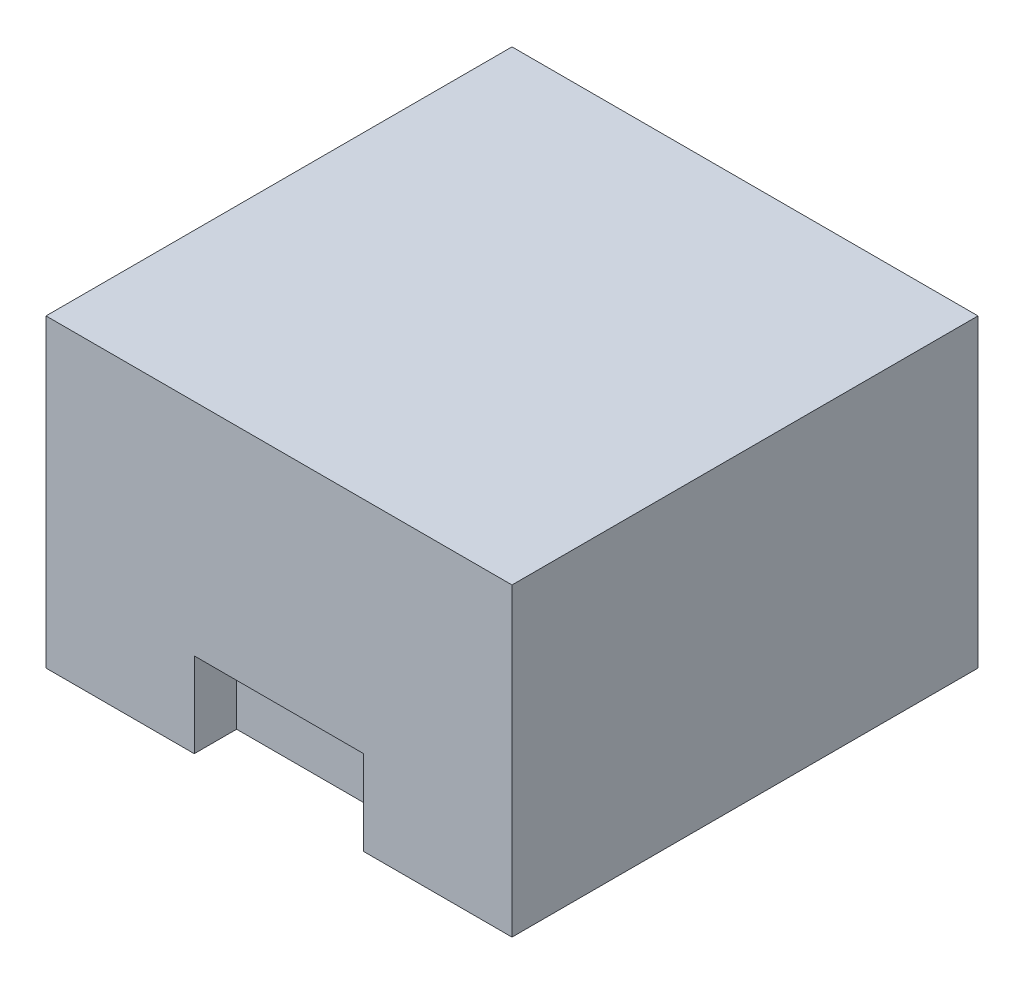
SolidWorks part; units mm, degrees
ref_plane "Front Plane" through (0, 0, 0) normal (0, 0, 1) x (1, 0, 0)
ref_plane "Top Plane" through (0, 0, 0) normal (0, 1, 0) x (1, 0, 0)
ref_plane "Right Plane" through (0, 0, 0) normal (1, 0, 0) x (0, 0, -1)
sketch "Sketch1" plane through (0, 0, 0) normal (0, 1, 0) x (1, 0, 0)
  line L1 (-55, -55) -> (55, -55)
  line L2 (-55, -55) -> (-55, 55)
  line L3 (-55, 55) -> (55, 55)
  line L4 (55, -55) -> (55, 55)
  line L5 (-55, -55) -> (55, 55) construction
  line L6 (-55, 55) -> (55, -55) construction
  point P0 (0, 0)
  dimension "D1" = 110
  dimension "D2" = 110
extrude "Boss-Extrude1" add sketch "Sketch1" along normal blind 72
sketch "Sketch2" plane through (0, 0, 55) normal (0, 0, 1) x (1, 0, 0)
  line L0 (-55, 0) -> (55, 0) construction
  line L1 (-20, 0) -> (20, 0)
  line L2 (-20, 0) -> (-20, 20)
  line L3 (-20, 20) -> (20, 20)
  line L4 (20, 0) -> (20, 20)
  dimension "D1" = 40
  dimension "D2" = 20
  dimension "D3" = 20
extrude "Cut-Extrude1" cut sketch "Sketch2" against normal blind 10
